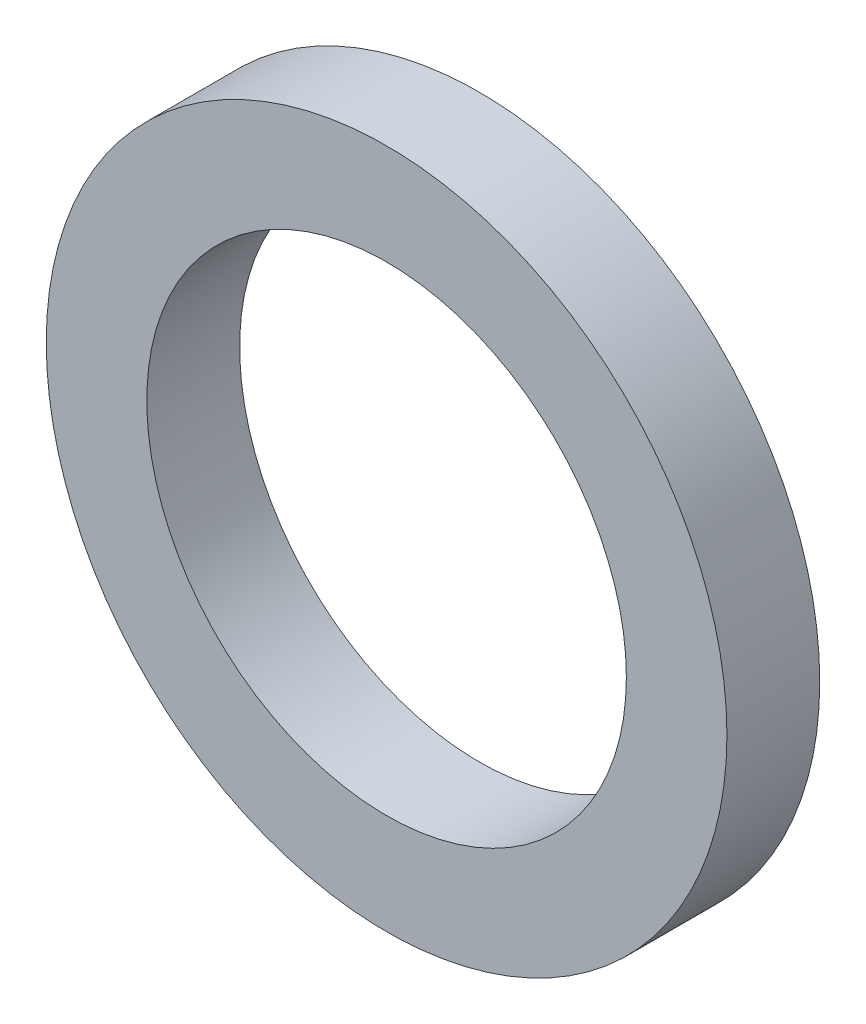
from build123d import *

# Parameters (mm, degrees)
SKETCH_1_R      = 11
SKETCH_1_R_2    = 7.75
EXTRUDE_1_DEPTH = 3


with BuildPart() as part:
    # 草图1 → 凸台-拉伸1 (new body)
    with BuildSketch(Plane.XY):
        Circle(SKETCH_1_R)
        Circle(SKETCH_1_R_2, mode=Mode.SUBTRACT)
    extrude(amount=EXTRUDE_1_DEPTH)


solid = part.part
